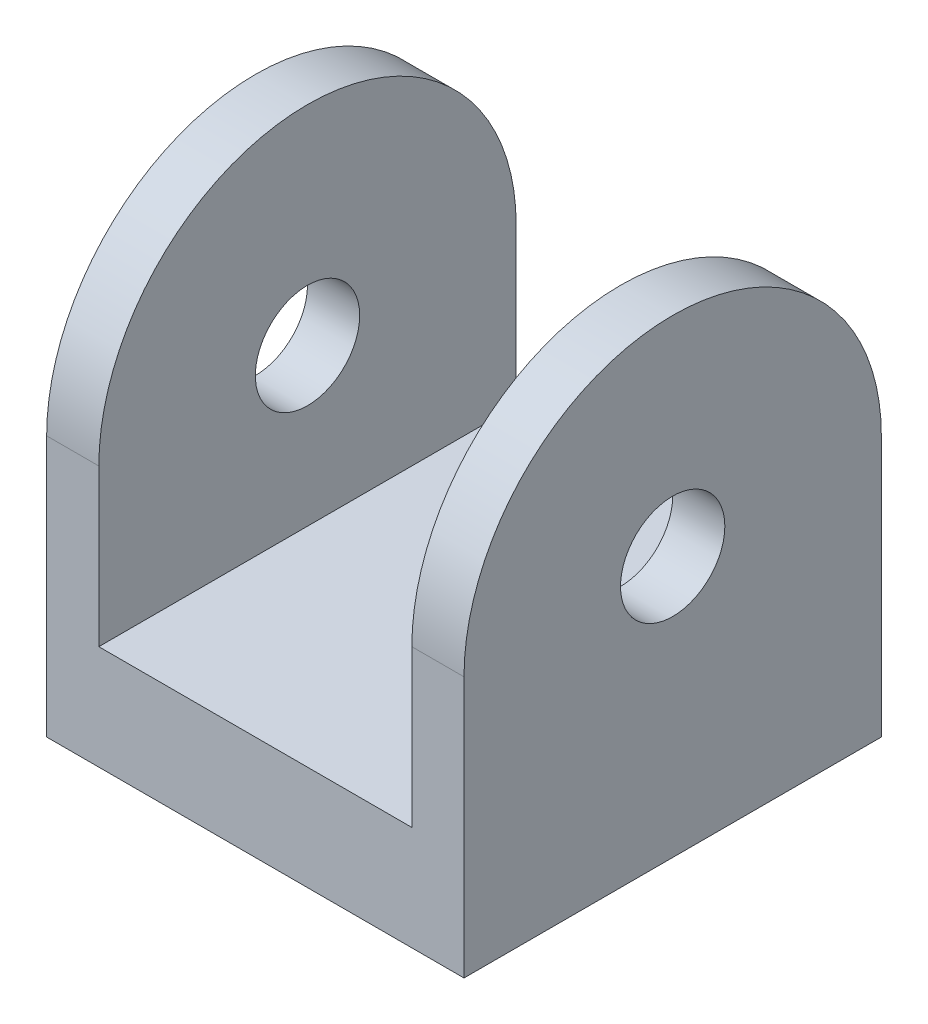
SolidWorks part; units mm, degrees
ref_plane "Front Plane" through (0, 0, 0) normal (0, 0, 1) x (1, 0, 0)
ref_plane "Top Plane" through (0, 0, 0) normal (0, 1, 0) x (1, 0, 0)
ref_plane "Right Plane" through (0, 0, 0) normal (1, 0, 0) x (0, 0, -1)
sketch "Sketch1" plane through (0, 0, 0) normal (0, 1, 0) x (1, 0, 0)
  line L1 (-20, 20) -> (20, 20)
  line L2 (-20, 20) -> (-20, -20)
  line L3 (-20, -20) -> (20, -20)
  line L4 (20, 20) -> (20, -20)
  line L5 (-20, 20) -> (20, -20) construction
  line L6 (-20, -20) -> (20, 20) construction
  point P0 (0, 0)
  dimension "D1" = 40
  dimension "D2" = 40
extrude "Boss-Extrude1" add sketch "Sketch1" along normal blind 10
sketch "Sketch2" plane through (20, 0, 0) normal (1, 0, 0) x (0, 0, -1)
  line L0 (0, 35.7483) -> (0, -19.103) construction
  line L5 (-20, 10) -> (-20, 25)
  line L6 (20, 10) -> (20, 25)
  line L7 (-20, 10) -> (20, 10)
  arc A0 (-20, 25) -> (20, 25) centre (0, 25) cw
  dimension "D1" = 15
extrude "Boss-Extrude2" add sketch "Sketch2" against normal blind 5
mirror "Mirror1" about plane through (0, 0, 0) normal (1, 0, 0) of "Boss-Extrude2"
ref_plane "Plane1" through (17.5, 0, 0) normal (1, 0, 0) x (0, 0, -1)
sketch "Sketch4" plane through (17.5, 0, 0) normal (1, 0, 0) x (0, 0, -1)
  circle A0 centre (0, 25) radius 5
  dimension "D1" = 10
extrude "Cut-Extrude1" cut sketch "Sketch4" against normal mid plane 105 contours A0
